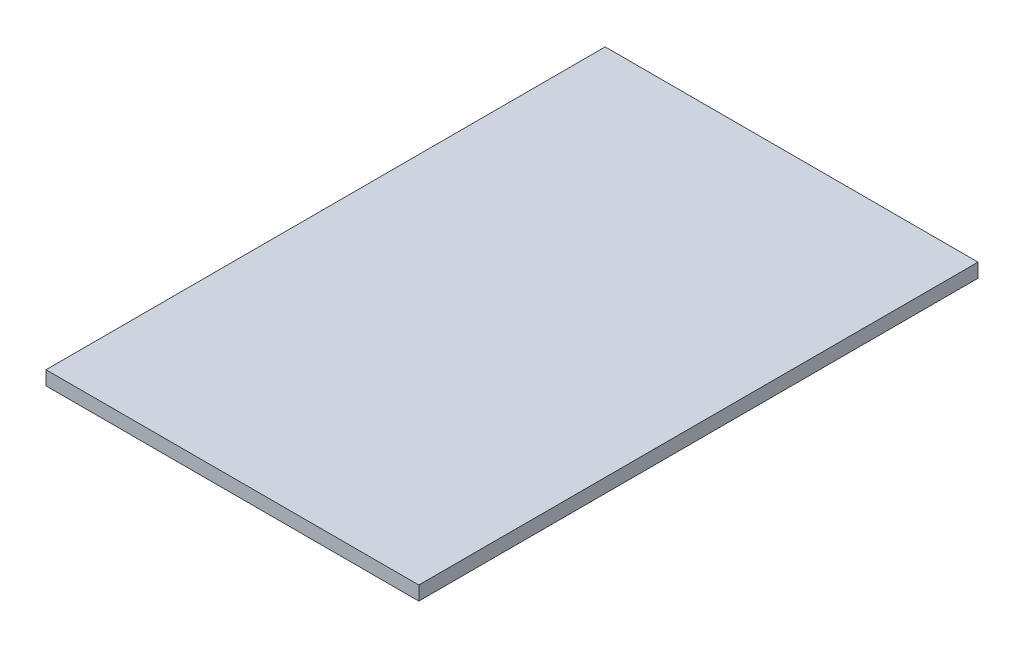
from build123d import *

# Parameters (mm, degrees)
SKETCH_1_W      = 800
SKETCH_1_H      = 1200
EXTRUDE_1_DEPTH = 30


with BuildPart() as part:
    # 草图1 → 凸台-拉伸1 (new body)
    with BuildSketch(Plane(origin=(0, 0, 0), x_dir=(1, 0, 0), z_dir=(0, 1, 0))):
        Rectangle(SKETCH_1_W, SKETCH_1_H)
    extrude(amount=EXTRUDE_1_DEPTH)


solid = part.part
